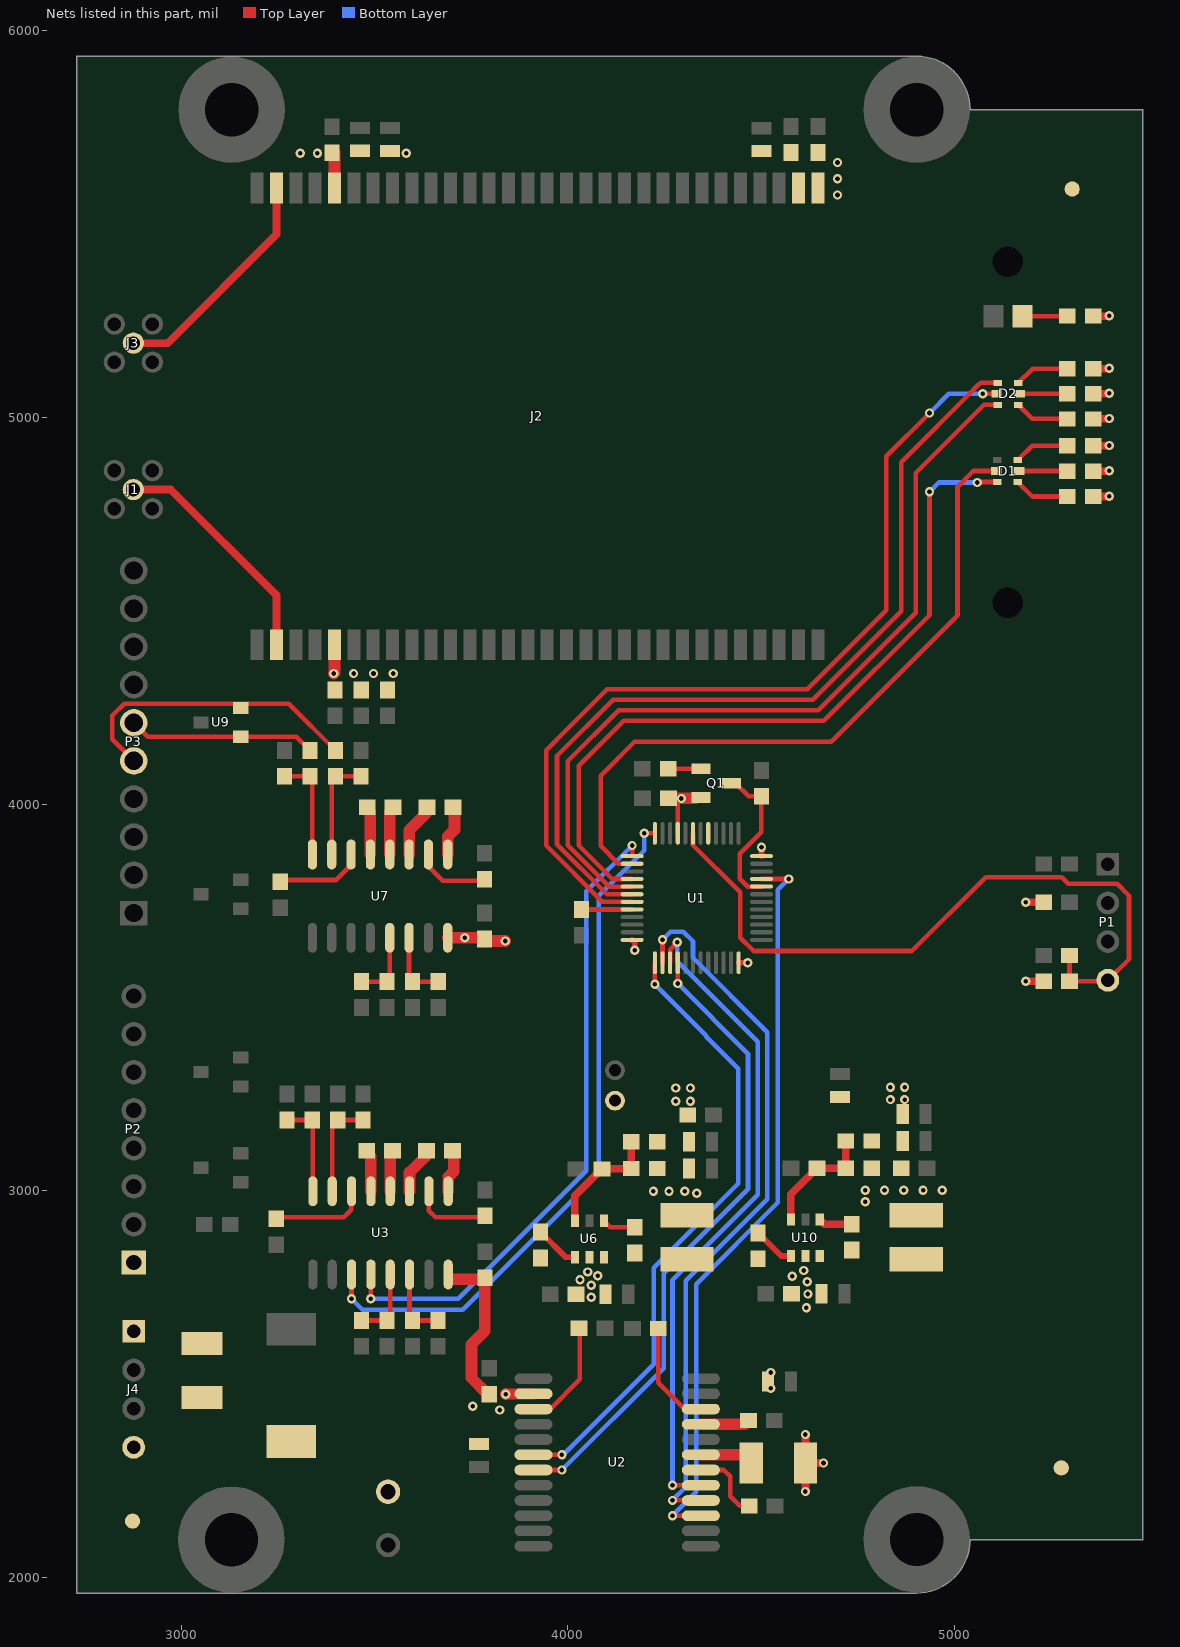
[diagram p0: the nets of this part, all layers, seen from the top]
# Altium PCB MISC84436.PcbDoc (part 2 of 2)
Units mil, origin at the board's own origin, x right, y up, seen from the top; angles counter-clockwise.
Board outline 2756.44 x 3974.35 mil, 4 copper layers (Top Layer, GND2, POWER3, Bottom Layer), stack 23.756 mil thick; 107 components, 89 nets, 422 pads, 390 vias.

## Via types
v1: diameter 24, hole 12, Top Layer to Bottom Layer, tented both sides, 252 vias
v2: diameter 24, hole 12, Top Layer to Bottom Layer, 138 vias

## Nets (pads, with @x,y where several pads share a name; then routed paths per layer and width w, separated by ;. In a path a pad name is that pad's centre, name@x,y a point inside that pad or via, vN(x,y) a via of type N, cw(c..) or ccw(c..) an arc to the next point about the centre after c; other vN are vias at no path point) (continued)
LED1_G: D1.1 U1.16 | length 1953
  Top Layer w12: U1.16@4165.76,3806.31 4114.56,3806.31 4027.87,3892.99 4027.87,4099.13 4144.27,4215.53 4661.59,4215.53 4935.04,4488.98 v1(4935.04,4807.48) ; v1(5058.11,4831.65) 5059.33,4832.87 D1.1@5110.43,4832.87
  Bottom Layer w12: v1(4935.04,4807.48) 4959.21,4831.65 v1(5058.11,4831.65)
LED1_R: D1.3 U1.14 | length 1826.8
  Top Layer w12: U1.14@4165.76,3845.68 4130.42,3845.68 4084.25,3891.85 4084.25,4073.62 4172.05,4161.42 4680.58,4161.42 5007.48,4488.32 5007.48,4820.87 5048.03,4861.42 D1.3@5107.48,4861.42
LED2_B: D2.5 U1.18 | length 2242.4
  Top Layer w12: 3971.26,3896.46 4100.78,3766.94 U1.18@4165.76,3766.94 ; 3971.5,3896.46 3971.5,4124.65 4116.49,4269.64 4633.02,4269.64 4861.81,4498.43 4861.81,4884.25 5048.44,5070.88 5048.44,5071.36 5062.5,5085.42 5062.98,5085.42 5067.13,5089.57 D2.5@5111.61,5089.57
LED2_G: D2.1 U1.17 | length 2133.5
  Top Layer w12: U1.17@4165.75,3786.63 4106.55,3786.63 3999.68,3893.49 3999.68,4111.5 4130.77,4242.58 4647.31,4242.58 4899.61,4494.88 4899.61,4856.3 5075.79,5032.48 D2.1@5111.61,5032.48
LED2_R: D2.3 U1.19 | length 2309.9
  Top Layer w12: U1.19@4165.75,3747.26 4088.97,3747.26 3943.31,3892.91 3943.31,4139.09 4001.34,4197.12 4100.91,4296.69 4618.74,4296.69 4823.23,4501.18 4823.23,4899.61 v1(4935.04,5011.42) ; v1(5072.44,5061.42) 5072.83,5061.02 D2.3@5108.66,5061.02
  Bottom Layer w12: v1(4935.04,5011.42) 4985.04,5061.42 v1(5072.44,5061.42)
MARK: 
MARK1: pad.MARK@5303.94,5590.55
MARK2: pad.MARK@2874.02,2145.67
MARK3: pad.MARK@5275.59,2283.46
MCU_DB_232RX: P3.6 R25.1 U9.1 | length 485.3
  Top Layer w12: P3.6@2877.17,4210.24 2913.39,4174.02 3148.43,4174.02 3297.49,4174.02 R25.1@3332.81,4138.7
MCU_DB_232TX: P3.5 R24.1 U9.2 | length 779.9
  Top Layer w12: P3.5@2877.17,4111.81 2821.65,4167.32 2821.65,4229.13 2851.97,4259.45 3277.94,4259.45 R24.1@3398.69,4138.7
NetC11_1: C11.1 U2.15 | length 284.2
  Top Layer w12: U2.15@3910.61,2435.43 3953.93,2435.43 4030.71,2512.2 C11.1@4030.71,2644.49
NetC12_1: C12.1 U2.10 | length 278.2
  Top Layer w12: C12.1@4233.76,2643.7 4233.76,2503.64 4301.98,2435.43 U2.10@4343.69,2435.43
NetC13_1: C13.1 U2.6 | length 193.7
  Top Layer w12: U2.6@4343.69,2277.94 4403.16,2277.94 4419.29,2261.81 4419.29,2210.24 4444.09,2185.43 C13.1@4468.9,2185.43
NetC18_1: C18.1 U3.3 | length 121.4
  Top Layer w30: U3.3@3590.16,2998.86 3590.16,3047.24 3630.16,3087.24 C18.1@3630.16,3103.66
NetC18_2: C18.2 U3.1 | length 110.9
  Top Layer w30: U3.1@3690.16,2998.86 3690.16,3035.83 3704.96,3050.63 C18.2@3704.96,3103.66
NetC20_1: C20.1 U3.2 | length 202.6
  Top Layer w12: U3.2@3640.16,2998.86 3640.16,2948.43 3657.42,2931.16 C20.1@3785.16,2931.16
NetC21_1: C21.1 U3.5 | length 110.9
  Top Layer w30: C21.1@3475.35,3103.66 3490.16,3088.86 U3.5@3490.16,2998.86
NetC21_2: C21.2 U3.4 | length 108.9
  Top Layer w30: U3.4@3540.16,2998.86 3540.16,3093.66 C21.2@3550.16,3103.66
NetC22_2: C22.2 R14.2 U3.14 | length 188
  Top Layer w12: U3.14@3590.16,2783.46 3590.16,2672.22 R14.2@3597.77,2664.61 C22.2@3663.78,2664.61
NetC23_2: C23.2 R16.2 U3.13 | length 188.3
  Top Layer w12: C23.2@3465.75,2664.61 R16.2@3531.76,2664.61 3540.16,2673.01 U3.13@3540.16,2783.46
NetC24_1: C24.1 U3.6 | length 250.2
  Top Layer w12: C24.1@3245.32,2931.54 3419.72,2931.54 3439.37,2951.18 3439.37,2998.07 U3.6@3440.16,2998.86
NetC26_1: C26.1 R18.2 U3.8 | length 250.4
  Top Layer w12: C26.1@3273.23,3183.07 R18.2@3338.85,3183.07 3340.16,3181.76 U3.8@3340.16,2998.86
NetC27_1: C27.1 R17.2 U3.7 | length 255.8
  Top Layer w12: U3.7@3390.16,2998.86 3390.16,3168.77 R17.2@3404.46,3183.07 C27.1@3470.08,3183.07
NetC28_1: C28.1 L3.1 U6.6
NetC28_2: C28.2 U6.1 | length 87.2
  Top Layer w12: U6.1@4092.59,2922.56 4109.4,2905.75 C28.2@4172.83,2905.75
NetC29_2: C29.2 R19.1 R21.2 U6.3 | length 308.8
  Top Layer w20: U6.3@4017.79,2922.56 4017.79,2986.72 R21.2@4087.72,3056.65 4163.07,3056.65 R19.1@4163.7,3057.28 C29.2@4163.7,3126.8
NetC36_1: C36.1 U7.3 | length 139.8
  Top Layer w30: U7.3@3588.98,3869.72 3588.98,3932.68 3631.57,3975.28 C36.1@3631.57,3991.83
NetC36_2: C36.2 U7.1 | length 129.3
  Top Layer w30: U7.1@3688.98,3869.72 3688.98,3916.14 3706.38,3933.54 C36.2@3706.38,3991.83
NetC38_1: C38.1 U7.2 | length 191.1
  Top Layer w12: U7.2@3638.98,3869.72 3638.98,3838.98 3675.93,3802.03 C38.1@3783.98,3802.03
NetC39_1: C39.1 U7.5 | length 127.2
  Top Layer w30: C39.1@3476.57,3991.83 3488.98,3979.43 U7.5@3488.98,3869.72
NetC39_2: C39.2 U7.4 | length 127.2
  Top Layer w30: U7.4@3538.98,3869.72 3538.98,3979.43 C39.2@3551.38,3991.83
NetC40_2: C40.2 R22.2 U7.14 | length 182.3
  Top Layer w12: U7.14@3588.98,3654.33 3588.98,3547.66 3594.13,3542.5 R22.2@3595.67,3544.04 ; R22.2@3598.02,3540.94 C40.2@3664.17,3540.94
NetC41_2: C41.2 R23.2 U7.13 | length 195.3
  Top Layer w12: C41.2@3461.75,3541.67 C41.2@3461.02,3540.94 ; R23.2@3527.99,3542.5 3538.98,3553.48 U7.13@3538.98,3654.33 ; R23.2@3531.88,3540.94 C41.2@3465.73,3540.94 ; C41.2@3461.02,3540.94 3460.22,3540.14 3464.92,3540.14 C41.2@3465.73,3540.94 ; C41.2@3461.02,3540.94 C41.2@3465.73,3540.94
NetC42_1: C42.1 U7.6 | length 219.1
  Top Layer w12: C42.1@3262.99,3803.58 3399.65,3803.58 3438.98,3842.91 U7.6@3438.98,3869.72
NetC43_1: C43.1 R25.2 U7.8 | length 262
  Top Layer w12: C43.1@3266.93,4071.77 R25.2@3332.81,4071.77 ; U7.8@3338.98,3869.72 R25.2@3338.98,4065.83
NetC44_1: C44.1 R24.2 U7.7 | length 258.9
  Top Layer w12: U7.7@3388.98,3869.72 R24.2@3388.98,4062.76 ; R24.2@3398.69,4071.77 C44.1@3464.57,4071.77
NetC45_1: C45.1 L4.1 U10.6
NetC45_2: C45.2 U10.1 | length 87.7
  Top Layer w20: U10.1@4651.1,2925.7 4663.34,2913.46 C45.2@4733.7,2913.46
NetC46_2: C46.2 R26.1 R29.2 U10.3 | length 305.5
  Top Layer w20: U10.3@4576.3,2925.7 4576.3,2991.06 R29.2@4643.7,3058.46 R26.1@4718.5,3058.46 C46.2@4718.5,3128.46
NetD1_2: D1.2 R8.2 | length 143.2
  Top Layer w12: D1.2@5163.58,4832.87 5200.98,4795.47 R8.2@5291.34,4795.47
NetD1_4: D1.4 R10.2 | length 125
  Top Layer w12: D1.4@5166.54,4861.42 5290.94,4861.42 R10.2@5291.34,4861.02
NetD1_6: D1.6 R12.2 | length 142.9
  Top Layer w12: D1.6@5163.58,4889.96 5200.2,4926.57 R12.2@5291.34,4926.57
NetD2_2: D2.2 R9.2 | length 141.6
  Top Layer w12: D2.2@5164.76,5032.48 5200.98,4996.26 R9.2@5291.34,4996.26
NetD2_4: D2.4 R11.2 | length 123.7
  Top Layer w12: D2.4@5167.72,5061.02 5291.14,5061.02 R11.2@5291.34,5061.22
NetD2_6: D2.6 R13.2 | length 141.7
  Top Layer w12: D2.6@5164.76,5089.57 5201.38,5126.18 R13.2@5291.34,5126.18
NetD4_1: D4.1 R27.1 | length 116.2
  Top Layer w12: D4.1@5175.2,5261.81 R27.1@5291.14,5261.81
  Top Layer w20: R27.1@5291.14,5261.81 R27.1@5291.34,5262.01
NetJ1_1: J1.1 J2.2 | length 611.2
  Top Layer w20: J1.1@2875.98,4813.39 2972.83,4813.39 3246.06,4540.16 J2.2@3246.06,4412.2
NetJ2_59: J2.59 J3.1 | length 606.4
  Top Layer w20: J3.1@2875.98,5192.13 2964.57,5192.13 3246.06,5473.62 J2.59@3246.06,5593.31
NetL1_2: L1.2 U2.7 | length 139.1
  Top Layer w30: U2.7@4343.69,2317.32 4452.76,2317.32 L1.2@4474.02,2296.06
NetQ1_1: Q1.1 R3.1 | length 84.6
  Top Layer w12: R3.1@4259.21,4091.5 4343.47,4091.5 Q1.1@4343.7,4091.73
NetQ1_3: Q1.3 R4.2 U1.44 | length 393
  Top Layer w12: Q1.3@4422.44,4054.33 4433.07,4054.33 4467.17,4020.24 R4.2@4500.16,4020.24 4500.16,3927.72 4444.09,3871.65 4444.09,3807.09 4464.56,3786.62 U1.44@4500.39,3786.62
NetR20_1: R20.1 U6.4 | length 115.7
  Top Layer w15: R20.1@3929.13,2893.31 3994.37,2828.07 U6.4@4017.79,2828.07
NetR28_1: R28.1 U10.4 | length 118.8
  Top Layer w15: R28.1@4491.73,2890.94 4551.46,2831.22 U10.4@4576.3,2831.22 U10.4@4566.82,2831.22
NRST: C14.2 P1.4 R5.1 U1.7 | length 1847.2
  Top Layer w12: U1.7@4323.24,3924.41 4323.24,3894.08 4445.67,3771.65 4445.67,3654.85 4480.44,3620.08 4889.37,3620.08 5080.31,3811.02 5276.77,3811.02 5293.7,3794.09 5420.08,3794.09 5450.79,3763.39 5450.79,3599.21 P1.4@5396.06,3544.49 5393.31,3541.73 R5.1@5297.09,3541.73 C14.2@5297.09,3608.66
PB2_BOOT1: R1.2 U1.20 | length 130.7
  Top Layer w12: R1.2@4035.04,3727.56 U1.20@4165.76,3727.57
SCC_CLK: U1.26 U2.4 | length 1857.8
  Top Layer w12: U1.26@4244.5,3589.78 v2(4244.5,3649.2) ; v1(4270.09,2199.2) U2.4@4343.69,2199.2
  Bottom Layer w12: v2(4244.5,3649.2) 4265.16,3669.86 4298.25,3669.86 4323.23,3644.88 4323.23,3602.76 4515.75,3410.24 4515.75,2977.95 4304.72,2766.93 4304.72,2233.84 v1(4270.09,2199.2)
SCC_CS: U1.25 U2.18 | length 1626.4
  Top Layer w12: U2.18@3910.61,2317.32 v1(3984.21,2317.32) ; v2(4224.8,3533.86) U1.25@4224.8,3589.78
  Bottom Layer w12: v1(3984.21,2317.32) 3988.18,2317.32 4222.05,2551.18 4222.05,2800.79 4440.16,3018.9 4440.16,3315.74 4357.48,3398.42 4357.48,3401.18 v2(4224.8,3533.86)
SCC_MISO: U1.27 U2.5 | length 2035
  Top Layer w12: U1.27@4264.17,3589.78 4264.17,3624.02 v2(4282.68,3642.52) ; v1(4270.08,2238.58) U2.5@4343.69,2238.57
  Bottom Layer w12: v1(4270.08,2238.58) 4270.08,2338.58 ; 4270.08,2657.87 4270.08,2338.58 ; v2(4282.68,3642.52) 4282.68,3593.69 4490.94,3385.43 4490.94,2989.76 4270.08,2768.9 4270.08,2338.58
SCC_MOSI: U1.28 U2.19 | length 1659.9
  Top Layer w12: U2.19@3910.61,2277.94 v1(3984.21,2277.94) ; v2(4283.87,3536.23) U1.28@4283.87,3589.78
  Bottom Layer w12: v1(3984.21,2277.94) 4247.24,2540.98 4247.24,2786.22 4465.35,3004.33 4465.35,3354.74 v2(4283.87,3536.23)
SCC_RST: U1.45 U2.3 | length 1915.1
  Top Layer w12: v1(4270.09,2159.83) U2.3@4343.69,2159.83 ; U1.45@4500.4,3806.3 v2(4570.87,3806.3)
  Bottom Layer w12: v1(4270.09,2159.83) 4331.49,2221.24 4331.49,2758.26 4542.91,2969.68 4542.91,3778.35 v2(4570.87,3806.3)
UART2_RXD: U1.13 U3.12 | length 1674.3
  Top Layer w12: v1(3490.16,2720.91) U3.12@3490.16,2783.46 ; U1.13@4165.75,3865.37 v1(4165.75,3892.91)
  Bottom Layer w12: v1(3490.16,2720.91) 3716.18,2720.91 4047.24,3051.97 4047.24,3774.4 v1(4165.75,3892.91)
UART2_TXD: U1.12 U3.11 | length 1815.9
  Top Layer w12: v1(3440.16,2720.91) U3.11@3440.16,2783.46 ; v1(4197.26,3924.41) U1.12@4224.8,3924.41
  Bottom Layer w12: v1(3440.16,2720.91) 3468.54,2692.52 3727.95,2692.52 4079.92,3044.49 4079.92,3762.6 4197.26,3879.94 v1(4197.26,3924.41)
VDD_3.3: C1.1 C2.1 C9.1 C10.1 C15.2 C16.2 C17.2 C19.1 C37.1 C46.1 C47.1 C48.1 C49.1 C50.1 J2.31 J2.32 J4.4 L1.1 L4.2 Q1.2 R2.2 R5.2 R7.2 R8.1 R9.1 R10.1 R11.1 R12.1 R13.1 R26.2 R27.2 U1.9 U1.24 U1.36 U1.48 U2.9 U2.14 U3.16 U7.16 | length 1586.3
  Top Layer w12: R2.2@4259.61,4015.12 4275.2,4015.12 4283.87,4006.45 U1.9@4283.87,3924.41
  Top Layer w15: U1.24@4165.76,3648.83 4172.44,3642.14 v1(4172.44,3622.05) ; U1.36@4441.35,3589.78 v1(4464.57,3589.76) ; U1.48@4500.39,3865.36 v1(4500.39,3888.19)
  Top Layer w20: v1(4614.02,2222.46) L1.1@4614.02,2296.06 ; v1(4614.02,2369.66) L1.1@4614.02,2296.06 ; v1(4660.72,2296.06) L1.1@4614.02,2296.06 ; v1(5183.46,3541.73) R5.2@5230.16,3541.73 ; v1(5183.46,3746.06) R7.2@5230.16,3746.06 ; R8.1@5358.27,4795.47 v1@5399.61,4795.47 ; R10.1@5358.27,4861.02 v1@5399.61,4861.02 ; R12.1@5358.27,4926.57 v1@5399.61,4926.57 ; R9.1@5358.27,4996.26 v1@5399.61,4996.26 ; R11.1@5358.27,5061.22 v1@5399.61,5061.22 ; R13.1@5358.27,5126.18 v1@5399.61,5126.18 ; R27.2@5358.27,5262.01 v1@5399.61,5262.01
  Top Layer w28: v1@3839.76,2474.8 U2.14@3910.61,2474.8
  Top Layer w30: U7.16@3688.98,3654.33 v1(3732.87,3654.33) 3776.77,3654.33 3785.04,3646.06 v1(3837.4,3646.06) ; 3702.46,2771.16 C19.1@3785.16,2771.16 ; C19.1@3785.16,2775.1 C19.1@3785.16,2771.16 ; C10.1@3796.46,2474.02 3792.35,2474.02 3750.39,2515.97 3750.39,2602.76 3785.16,2637.52 C19.1@3785.16,2771.16 ; v1(3838.98,2474.02) v1@3839.76,2474.8 ; R2.2@4275.2,4015.12 Q1.2@4328.9,4015.12 ; U2.9@4343.69,2396.06 4456.69,2396.06 C9.1@4466.54,2405.91
  other v1: 3823.23,2433.07 3753.54,2442.52 4524.02,2489.37 4524.02,2529.92 4768.9,2971.65 4768.9,3001.57 4818.7,3001.57 4868.5,3001.57 4918.31,3001.57 4968.11,3001.57 4833.86,3235.83 4870.47,3235.83 4833.86,3267.72 4870.47,3267.72 4293.31,4014.57 5399.61,4796.46 5399.61,4862.01 5399.61,4927.56 5399.61,4997.24 5399.61,5062.2 5399.61,5127.17 5399.61,5262.99 4696.85,5575.39 4696.85,5617.32 4696.85,5659.25
VDD_5V: C3.2 C4.2 C5.1 C6.1 C7.2 C8.2 C29.1 C30.1 C31.1 C32.1 C33.1 J2.5 J2.56 L3.2 R19.2 | length 167.4
  Top Layer w30: v1(3394.09,4337.8) 3396.06,4339.76 J2.5@3396.06,4412.2 ; J2.56@3396.06,5593.31 C5.1@3396.06,5685.43
  other v1: 4332.68,2993.31 4220.87,2998.82 4261.29,2998.82 4301.71,2998.82 4278.74,3231.5 4316.54,3231.5 4278.35,3265.75 4316.54,3265.75 3445.54,4337.8 3496.98,4337.8 3548.42,4337.8 3307.48,5683.07 3351.97,5683.07 3581.89,5683.46
VDD_12V: C25.1 C34.2 C35.2 C51.2 C52.2 D3.2 R15.1 R20.2 R28.2 U6.5 U10.5
  other v2: 4616.54,2697.24 4060.24,2724.8 4620.47,2733.07 4060.24,2755.91 4618.5,2764.57 4031.1,2770.08 4579.92,2779.13 4076.77,2779.92 4050.79,2790.16 4609.84,2793.7
VDD_IN: J4.1 P2.1 R15.2
XTAL1: U1.5
pads on no net: J2.7 J2.8 J2.10 J2.11 J2.12 J2.13 J2.15 J2.16 J2.17 J2.19 J2.20 J2.21 J2.22 J2.23 J2.24 J2.26 J2.27 J2.28 J2.29 J2.30 J2.41 J2.42 J2.44 J2.45 J2.46 J2.48 J2.49 J2.50 J2.51 J2.53 J2.54 U1.1 U1.2 U1.3 U1.4 U1.6 U1.10 U1.11 U1.29 U1.32 U1.33 U1.38 U1.39 U1.40 U1.41 U1.42 U1.43 U1.46 U2.2 U2.11 U2.20 U2.21 U2.22 U2.23

## Polygon pours and split planes (outlines as drawn)
VDD_12V on Top Layer "BottomLayer-No Net" (solid, remove dead copper): 4450.39,2822.44 4450.39,2790.16 4457.87,2782.68 4465.35,2775.2 4491.34,2775.2 4536.61,2775.2 4547.64,2764.17 4553.54,2758.27 4553.54,2737.8 4553.54,2700.39 4559.84,2694.09 4574.02,2679.92 4584.65,2679.92 4655.51,2679.92 4662.99,2687.4 4674.41,2698.82 4674.41,2713.39 4674.41,2756.3 4663.78,2766.93 4627.56,2803.15 4627.56,2831.89 4627.56,2845.67 4624.02,2849.21 4622.44,2850.79 4616.54,2850.79 4604.33,2850.79 4602.36,2848.82 4601.97,2848.43 4601.97,2841.73 4601.97,2810.63 4593.31,2801.97 4585.04,2793.7 4566.54,2793.7 4542.52,2793.7 4521.65,2814.57 4514.57,2821.65 4514.57,2829.13 4514.57,2842.13 4510.63,2846.06 4506.3,2850.39 4483.86,2850.39 4469.69,2850.39 4457.48,2838.19 4450.39,2831.1 4450.39,2822.44
VDD_12V on Top Layer "BottomLayer-No Net" (solid, remove dead copper): 3898.03,2818.9 3898.03,2790.94 3906.69,2782.28 3913.78,2775.2 3937.4,2775.2 3977.56,2775.2 3988.19,2764.57 3996.85,2755.91 3996.85,2735.04 3996.85,2711.42 4001.18,2707.09 4007.09,2701.18 4026.77,2701.18 4110.63,2701.18 4112.6,2703.15 4117.32,2707.87 4117.32,2718.11 4117.32,2757.48 4068.5,2806.3 4067.72,2807.09 4067.72,2827.56 4067.72,2842.13 4065.35,2844.49 4064.57,2845.28 4059.06,2845.28 4046.46,2845.28 4044.09,2842.91 4043.31,2842.13 4043.31,2838.58 4043.31,2807.09 4040.94,2804.72 4035.43,2799.21 4024.41,2799.21 3979.13,2799.21 3962.6,2815.75 3957.87,2820.47 3957.87,2833.46 3957.87,2840.16 3950.39,2847.64 3948.43,2849.61 3938.98,2849.61 3911.81,2849.61 3904.33,2842.13 3898.03,2835.83 3898.03,2818.9
VDD_12V on Top Layer "BottomLayer-No Net" (solid, remove dead copper): 2972.83,2470.08 2972.83,2361.42 3016.54,2317.72 3035.83,2298.43 3113.39,2298.43 3240.94,2298.43 3313.78,2225.59 3361.81,2177.56 3503.94,2177.56 3560.63,2177.56 3577.56,2194.49 3589.37,2206.3 3589.37,2247.24 3589.37,2316.14 3552.76,2352.76 3489.76,2415.75 3400.79,2415.75 3352.36,2415.75 3310.63,2457.48 3261.02,2507.09 3134.65,2507.09 2996.85,2507.09 2977.56,2487.8 2972.83,2483.07 2972.83,2470.08
VDD_IN on Top Layer "BottomLayer-No Net" (solid, remove dead copper): 2817.72,2801.97 2817.72,2737.8 2817.72,2629.92 2844.49,2603.15 2846.46,2601.18 2897.64,2601.18 2955.12,2601.18 2975.98,2580.32 2988.19,2568.11 3034.25,2568.11 3102.76,2568.11 3114.96,2580.32 3120.08,2585.43 3120.08,2629.13 3120.08,2694.09 3045.28,2768.9 2959.84,2854.33 2900.79,2854.33 2848.03,2854.33 2833.46,2839.76 2817.72,2824.02 2817.72,2801.97
GND on Top Layer "Top Layer-GND 1" (solid, remove dead copper, pour order 46): 2742.34,1946.21 2742.61,1946.47 2742.61,5920.29 5360.45,5920.29 5498.51,5782.23 5498.51,2084.01 5360.72,1946.21
VDD_3.3 on Top Layer "Top Layer-VDD_3.3" (solid, remove dead copper, pour order 18): 3948.03,2497.64 3792.52,2497.64 3738.58,2443.7 3738.58,2343.31 3756.69,2325.2 3795.67,2325.2 3810.24,2339.76 3810.24,2397.64 3868.9,2456.3 3953.94,2456.3 3959.84,2462.2 3959.84,2485.83
GND on Top Layer "Top Layer-GND" (solid, remove dead copper, pour order 42): 4592.37,2981.49 4609.69,2998.82 4635.68,2998.81 4640.8,2993.7 4640.8,2970.86 4633.31,2963.38 4633.31,2873.22 4619.14,2859.05 4553,2859.05 4538.83,2873.22 4538.83,2888.58 4552.61,2902.36 4582.92,2902.36 4592.37,2911.81
GND on Top Layer "Top Layer-GND" (solid, remove dead copper, pour order 34): 4033.86,2978.35 4051.18,2995.67 4077.17,2995.67 4082.28,2990.55 4082.28,2967.72 4074.8,2960.24 4074.8,2870.08 4060.63,2855.91 3994.49,2855.91 3980.32,2870.08 3980.32,2885.43 3994.09,2899.21 4024.41,2899.21 4033.86,2908.66
VDD_5V on Top Layer "Top Layer-VDD_5V" (solid, remove dead copper, pour order 32): 3369.68,5554.72 3375.59,5548.82 3418.5,5548.82 3422.44,5552.76 3422.44,5638.98 3430.71,5647.24 3604.72,5647.24 3610.24,5652.76 3610.24,5711.42 3605.12,5716.54 3375.2,5716.54 3289.37,5716.54 3284.25,5711.42 3284.25,5653.54 3290.55,5647.24 3361.02,5647.24 3369.68,5638.58
VDD_3.3 on Top Layer "Top Layer-VDD_3.3 3" (solid, remove dead copper, pour order 0): 4709.45,5714.57 4724.02,5700 4724.02,5558.66 4710.63,5545.28 4585.43,5545.28 4577.17,5553.54 4577.17,5634.25 4563.39,5648.03 4478.35,5648.03 4471.26,5655.12 4471.26,5707.87 4477.95,5714.57
VDD_5V on Top Layer "Top Layer-VDD_5V 1" (solid, remove dead copper, pour order 10): 3383.86,4266.93 3369.29,4281.5 3369.29,4451.97 3381.1,4463.78 3409.06,4463.78 3423.23,4449.61 3423.23,4364.17 3431.89,4355.51 3563.39,4355.51 3571.26,4347.64 3571.26,4273.23 3564.96,4266.93
VDD_3.3 on Top Layer "Top Layer-VDD_3.3 1" (solid, remove dead copper, pour order 20): 4486.22,2375.2 4499.21,2388.19 4499.21,2440.94 4538.19,2479.92 4538.19,2544.09 4526.77,2555.51 4438.58,2555.51 4426.38,2543.31 4426.38,2433.46 4409.45,2416.54 4299.61,2416.54 4290.55,2407.48 4290.55,2385.04 4300.39,2375.2
VDD_3.3 on Top Layer "Top Layer-VDD_3.3 2" (solid, remove dead copper, pour order 16): 4675.99,3185.04 4756.3,3104.72 4756.3,2959.06 4800,2915.35 4982.28,2915.35 5000.39,2933.46 5000.39,3001.18 4984.65,3016.93 4912.6,3016.93 4882.68,3046.85 4882.68,3272.05 4871.65,3283.07 4735.83,3283.07 4675.98,3223.23
VDD_5V on Top Layer "Top Layer-VDD_5V 2" (solid, remove dead copper, pour order 8): 4325.2,3284.25 4337.8,3271.65 4337.8,3025.98 4370.47,2993.31 4370.47,2918.5 4359.45,2907.48 4221.26,2907.48 4201.97,2926.77 4201.97,3075.59 4094.49,3183.07 4094.49,3205.91 4172.83,3284.25
NetC45_1 on Top Layer "Top Layer-NetC45_1" (solid, remove dead copper, pour order 14): 4640.94,2845.67 4662.99,2867.72 4972.44,2867.72 4999.61,2840.55 4999.61,2780.71 4990.16,2771.26 4687.4,2771.26 4640.94,2817.72
NetC28_1 on Top Layer "Top Layer-NetC28_1" (solid, remove dead copper, pour order 6): 4083.07,2819.68 4083.07,2845.67 4106.3,2868.9 4365.75,2868.9 4369.29,2865.35 4369.29,2807.09 4355.51,2793.31 4101.97,2793.31 4082.95,2812.33
GND on Bottom Layer "Bottom Layer-GND" (solid, remove dead copper, pour order 48): 2716.97,1969.03 2716.97,5942.58 2717.23,5942.85 5335.61,5942.85 5473.4,5805.05 5473.14,5804.79 5473.14,2106.82 5335.34,1969.03
GND on GND2 (split plane): 4920.14,5912.89 4938.19,5908.56 4955.35,5901.45 4971.18,5891.75 4985.3,5879.69 4997.36,5865.57 5007.06,5849.74 5014.01,5832.95 5019.57,5805.08 5019.59,5796.25 5019.78,5794.31 5019.97,5792.38 5019.98,5792.35 5019.98,5792.33 5020.55,5790.48 5021.11,5788.61 5021.13,5788.58 5021.13,5788.56 5022.05,5786.85 5022.97,5785.13 5022.99,5785.11 5023,5785.09 5024.23,5783.59 5025.47,5782.09 5025.49,5782.07 5025.5,5782.05 5027,5780.83 5028.51,5779.58 5028.53,5779.57 5028.55,5779.56 5030.27,5778.64 5031.98,5777.72 5032.01,5777.72 5032.03,5777.71 5033.9,5777.14 5035.75,5776.58 5035.78,5776.58 5035.8,5776.57 5037.73,5776.38 5039.67,5776.19 5466.07,5775.94 5465.81,2117.63 5039.69,2117.63 5037.73,2117.43 5035.8,2117.25 5035.79,2117.24 5035.77,2117.24 5033.9,2116.68 5032.03,2116.11 5032.01,2116.1 5032,2116.1 5030.28,2115.18 5028.55,2114.26 5028.54,2114.25 5028.52,2114.24 5027.01,2113 5025.5,2111.77 5025.49,2111.75 5025.48,2111.74 5024.24,2110.23 5023,2108.73 5022.99,2108.71 5022.98,2108.7 5022.06,2106.98 5021.13,2105.26 5021.13,2105.24 5021.12,2105.22 5020.55,2103.34 5019.98,2101.49 5019.98,2101.47 5019.98,2101.45 5019.78,2099.51 5019.59,2097.57 5019.57,2088.74 5014.01,2060.87 5007.06,2044.08 4997.36,2028.24 4985.3,2014.12 4971.18,2002.07 4955.35,1992.36 4938.19,1985.26 4920.14,1980.92 4906.26,1979.83 4901.46,1979.83 2749.83,1980.09 2750.1,5913.99 4906.26,5913.99
VDD_3.3 on POWER3 (split plane): 592 vertices, not listed, extent 2769.81,1999.8 5446.11,5894.41
VDD_5V on POWER3 (split plane): 214 vertices, not listed, extent 2769.8,2970.72 4402.91,5894.18
VDD_12V on POWER3 (split plane): 4151.53,2953.5 4153.62,2951.89 4156.05,2950.89 4158.66,2950.54 4357.87,2950.54 4360.48,2950.89 4362.92,2951.89 4365.01,2953.5 4412.99,3001.48 4427.91,2986.57 4430,2984.97 4431.42,2984.38 4432.43,2983.96 4435.04,2983.61 4566.69,2983.61 4729.28,2821.02 4729.28,2651.82 4660,2582.53 3818.9,2582.53 3816.29,2582.18 3815.07,2581.68 3813.85,2581.18 3811.77,2579.57 3647.99,2415.79 3646.38,2413.7 3645.38,2411.27 3645.03,2408.66 3645.03,2217.56 3597.4,2169.93 3367.56,2169.93 3196.31,2341.19 3196.31,3198.58 3906.45,3198.58

## Keep-outs
Keep-Out Layer:
  circle w0.5: c4901.63,2097.8 r137.8
  circle w0.5: c3129.97,5796.02 r137.8
  circle w0.5: c4901.63,5796.02 r137.8
  circle w0.5: c3129.97,2097.8 r137.8
  lines w0.5: 4901.63,5933.82 2730,5933.82 2730,1960 4901.63,1960 ccw(c4901.63,2097.8) 5039.42,2097.8 5485.91,2097.8 5485.91,5796.02 5039.42,5796.02

## Other copper
Top Layer:
  pour cut-out: 4414.57,4368.11 4625.59,4368.11 4630.71,4362.99 4630.71,4331.89 4616.14,4317.32 4406.3,4317.32 4402.76,4320.87 4402.76,4356.3
  pour cut-out: 3130.03,5543.31 4711.02,5543.31 4711.02,4474.41 3127.5,4474.41
POWER3 (plane layer: these items are gaps in the copper):
  lines w20: 2757.48,3208.66 3910.63,3208.66 4158.66,2960.63 4357.87,2960.63 4412.99,3015.75 ; 3186.22,3208.66 3186.22,2337.01 3363.39,2159.84 3601.57,2159.84 3655.12,2213.39 3655.12,2408.66 3818.9,2572.44 4664.17,2572.44 4739.37,2647.64 4739.37,2825.2 4570.87,2993.7 4435.04,2993.7 4412.99,3015.75 ; 3675.59,5937.8 3675.59,4158.66 3675.59,3670.87 3737.8,3608.66 4115.75,3608.66 4412.99,3311.42 4412.99,3015.75

## Silkscreen, mask and mechanical layers (free items; w line width, h text height)
Top Overlay:
  lines w6: 4254.33,3471.26 4269.29,3456.3 4269.29,3034.41 4262.17,3027.28 ; 4769.29,3468.5 4787.01,3450.79 4787.01,3388.58 4824.02,3351.57 4824.02,3035.51 4816.97,3028.46 ; 5389.76,4365.35 5409.84,4385.43 5409.84,5136.14 5389.8,5156.18
  text "VDD_IN" at 2937.01,2370.87 h40
  text "GND" at 2947.64,2322.44 h40
  text "ACIN" at 2939.37,2270.47 h40
  text "3.3V" at 2934.65,2218.5 h40
  text "Agr-Ctrl_2GS_V1" at 5198.03,1859.45 h50
Bottom Overlay:
  text "GND" at 3050.79,4580.71 h40
  text "GND" at 3050.79,4486.22 h40
  text "GND" at 3050.79,4387.01 h40
  text "GND" at 3050.79,4290.16 h40
  text "MCU_DB_232RX" at 3409.45,4188.58 h40
  text "MCU_DB_232TX" at 3409.45,4089.37 h40
  text "GND" at 3047.64,3992.13 h40
  text "BOOT0" at 3129.53,3897.64 h40
  text "JTCK" at 5321.26,3831.1 h40
  text "GPS_DB_232RX" at 3410.24,3800.79 h40
  text "JTMS" at 5324.8,3736.22 h40
  text "GPS_DB_232TX" at 3408.66,3698.03 h40
  text "GND" at 5315.35,3626.77 h40
  text "NRST" at 5313.78,3522.83 h40
  text "GND" at 3054.72,3482.28 h40
  text "GND" at 3051.57,3385.04 h40
  text "GPS_RTK_232RX" at 3448.43,3289.37 h40
  text "GPS_RTK_232TX" at 3447.64,3186.22 h40
  text "232RX0" at 3173.62,3089.76 h40
  text "232TX0" at 3175.2,2992.52 h40
  text "GND_IN" at 3173.62,2896.06 h40
  text "VDD_IN" at 3173.62,2790.94 h40
  text "VDD_IN" at 3168.9,2616.54 h40
  text "GND" at 3057.09,2514.96 h40
  text "ACIN" at 3089.76,2414.57 h40
  text "VDD_3.3" at 3209.84,2317.72 h40
Mechanical 15:
  circle w0.5: c3129.97,2097.8 r137.8
  circle w0.5: c3129.97,2097.8 r68.9
  circle w0.5: c4901.63,5796.02 r137.8
  circle w0.5: c4901.63,5796.02 r68.9
  circle w0.5: c3129.97,5796.02 r68.9
  circle w0.5: c3129.97,5796.02 r137.8
  circle w0.5: c4901.63,2097.8 r68.9
  circle w0.5: c4901.63,2097.8 r137.8
  lines w0.5: 4888.38,4961.37 5324.97,4961.37 ; 5023.66,5161.77 5252.01,5161.77 ; 5137.83,4559.8 5137.83,5362.95 ; 2730,1960 4901.63,1960 ccw(c4901.63,2097.8) 5039.42,2097.8 5485.91,2097.8 5485.91,5796.02 5039.42,5796.02 ccw(c4901.63,5796.02) 4901.63,5933.82 2730,5933.82 2730,1960 ; 4988.56,4474.88 5483.88,4474.88 5483.88,5465.51 4988.56,5465.51 4988.56,4474.88 ; 5023.66,4631.26 5023.66,4690.31 5092.56,4690.31 5092.56,4631.26 5023.66,4631.26 ; 5023.66,4831.65 5023.66,4890.71 5092.56,4890.71 5092.56,4831.65 5023.66,4831.65 ; 5023.66,5032.04 5023.66,5091.1 5092.56,5091.1 5092.56,5032.04 5023.66,5032.04 ; 5023.66,5232.44 5023.66,5291.49 5092.56,5291.49 5092.56,5232.44 5023.66,5232.44 ; 5118.15,4481.06 cw(c5118.15,4520.43) 5118.15,4559.8 5157.52,4559.8 cw(c5157.52,4520.43) 5157.52,4481.06 5118.15,4481.06 ; 5118.15,5362.95 cw(c5118.15,5402.32) 5118.15,5441.69 5157.52,5441.69 cw(c5157.52,5402.32) 5157.52,5362.95 5118.15,5362.95 ; 5183.11,4631.26 5252.01,4631.26 5252.01,4690.31 5183.11,4690.31 5183.11,4631.26 ; 5183.11,4831.65 5183.11,4890.71 5252.01,4890.71 5252.01,4831.65 5183.11,4831.65 ; 5183.11,5032.04 5252.01,5032.04 5252.01,5091.1 5183.11,5091.1 5183.11,5032.04 ; 5183.11,5232.44 5252.01,5232.44 5252.01,5291.49 5183.11,5291.49 5183.11,5232.44